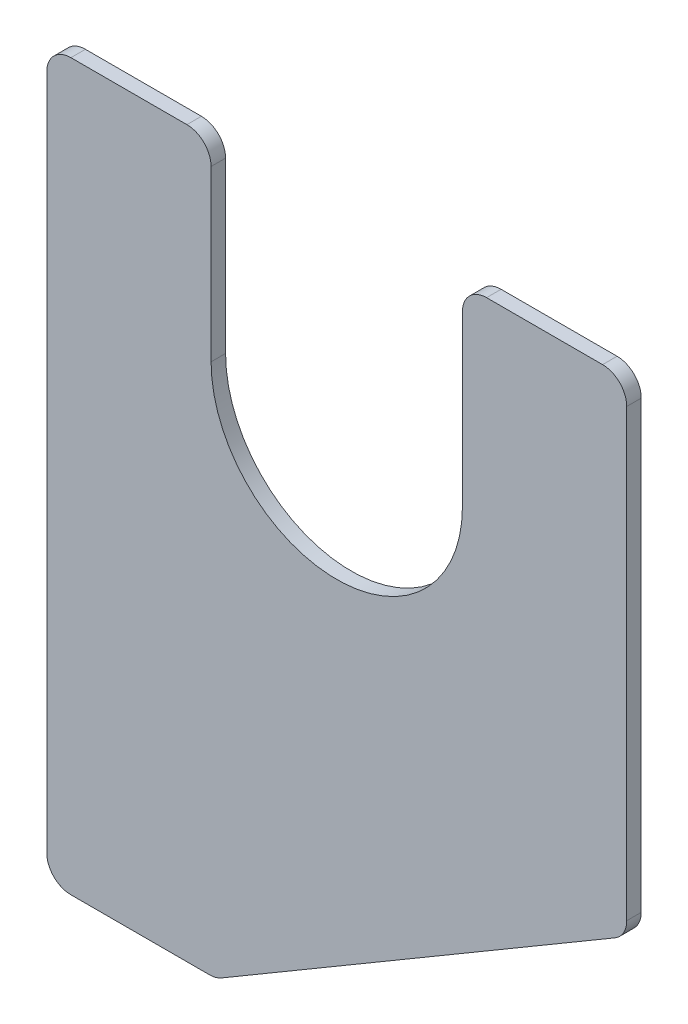
from build123d import *

# Parameters (mm, degrees)
BOSS_EXTRUDE1_DEPTH = 3


with BuildPart() as part:
    # Sketch1 → Boss-Extrude1 (new body)
    with BuildSketch(Plane.XY):
        with BuildLine():
            Line((0, -5), (0, -145))
            ThreePointArc((0, -145), (1.464466094, -148.535533906), (5, -150))
            Line((5, -150), (33.638458538, -150))
            ThreePointArc((33.638458538, -150), (34.952164103, -149.824331839), (36.173559171, -149.309671076))
            Line((36.173559171, -149.309671076), (117.535100633, -101.449940804))
            ThreePointArc((117.535100633, -101.449940804), (119.340247871, -99.622657373), (120, -97.140269728))
            Line((120, -97.140269728), (120, -5))
            ThreePointArc((120, -5), (118.535533906, -1.464466094), (115, 0))
            Line((115, 0), (91, 0))
            ThreePointArc((91, 0), (87.464466094, -1.464466094), (86, -5))
            Line((86, -5), (86, -40))
            ThreePointArc((86, -40), (60, -66), (34, -40))
            Line((34, -40), (34, -5))
            ThreePointArc((34, -5), (32.535533906, -1.464466094), (29, 0))
            Line((29, 0), (5, 0))
            ThreePointArc((5, 0), (1.464466094, -1.464466094), (0, -5))
        make_face()
    extrude(amount=BOSS_EXTRUDE1_DEPTH)


solid = part.part
